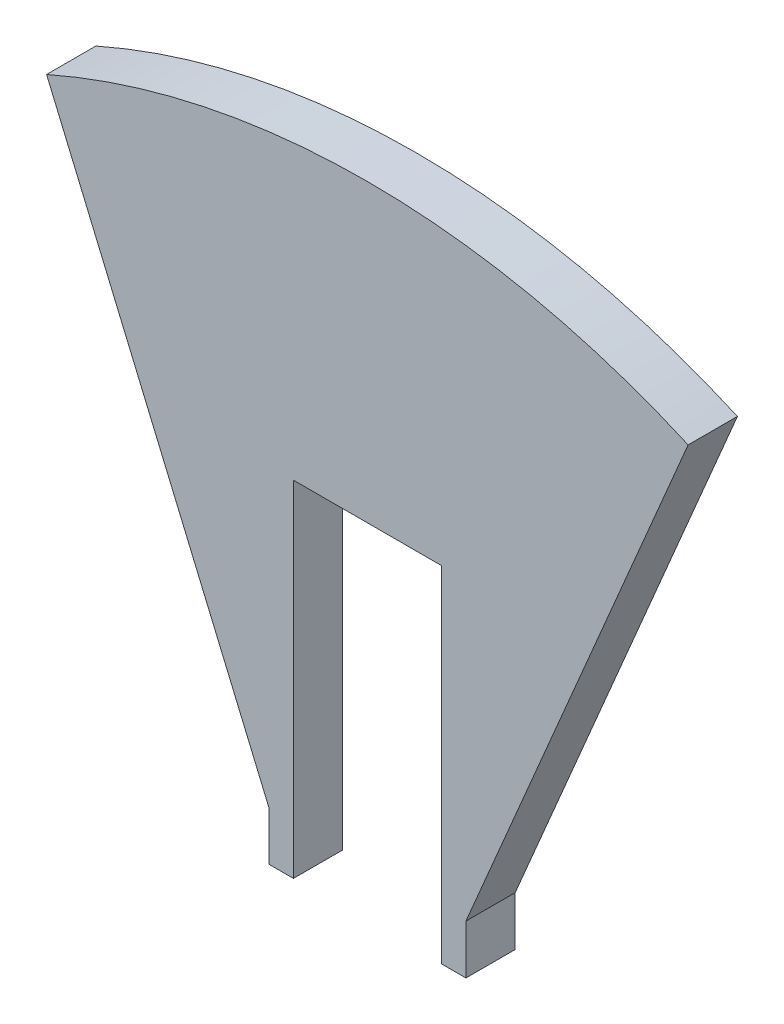
SolidWorks part; units mm, degrees
ref_plane "Front Plane" through (0, 0, 0) normal (0, 0, 1) x (1, 0, 0)
ref_plane "Top Plane" through (0, 0, 0) normal (0, 1, 0) x (1, 0, 0)
ref_plane "Right Plane" through (0, 0, 0) normal (1, 0, 0) x (0, 0, -1)
sketch "Sketch1" plane through (0, 0, 0) normal (0, 0, 1) x (1, 0, 0)
  line L0 (-65.1009, 147.2511) -> (-20, 41)
  line L1 (-20, 41) -> (-20, 31)
  line L2 (-20, 31) -> (20, 31)
  line L3 (20, 31) -> (20, 41)
  line L4 (20, 41) -> (65.1009, 147.2511)
  line L5 (0, 161) -> (0, 0) construction
  line L8 (15, 31) -> (15, 101)
  line L9 (15, 101) -> (-15, 101)
  line L10 (-15, 31) -> (-15, 101)
  line L11 (0, 31) -> (-15, 101) construction
  line L12 (15, 101) -> (0, 31) construction
  arc A0 (65.1009, 147.2511) -> (-65.1009, 147.2511) centre (0, 0) ccw
  point P1 (0, 31)
  dimension "D2" = 322
  dimension "D1" = 40
  dimension "D3" = 46
  dimension "D4" = 31
  dimension "D5" = 10
  dimension "D6" = 30
  dimension "D7" = 70
extrude "Boss-Extrude2" add sketch "Sketch1" along normal mid plane 10 contours L4 A0 L0 L1 L2 L10 L9 L8 L3
